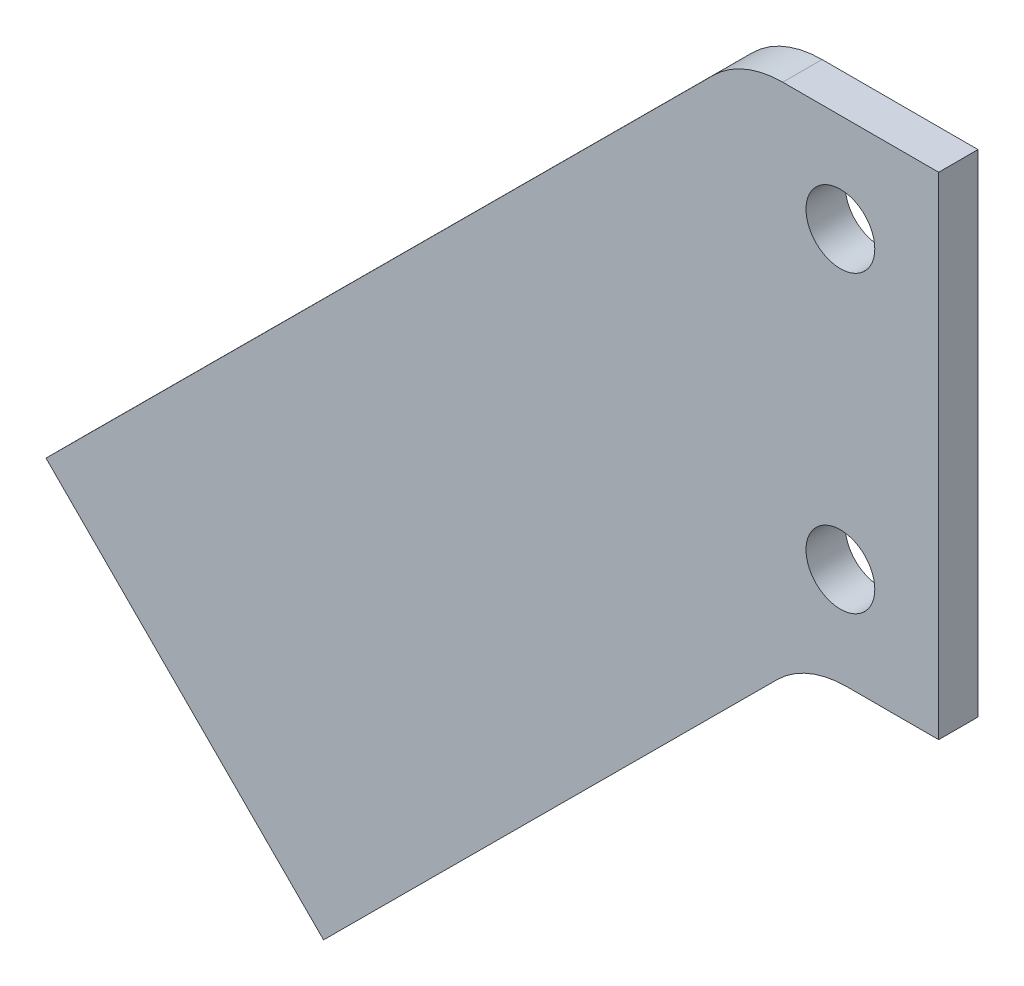
from build123d import *

# Parameters (mm, degrees)
SKETCH1_R           = 7
BOSS_EXTRUDE1_DEPTH = 8


with BuildPart() as part:
    # Sketch1 → Boss-Extrude1 (new body)
    with BuildSketch(Plane.XY):
        with BuildLine():
            Line((0, 0), (-31.73420201, 0))
            ThreePointArc((-31.73420201, 0), (-39.373295872, -1.516379008), (-45.854013577, -5.835575504))
            Line((-45.854013577, -5.835575504), (-181.644244963, -141.198115671))
            Line((-181.644244963, -141.198115671), (-125.164998695, -197.855813656))
            Line((-125.164998695, -197.855813656), (-32.854013577, -105.835575504))
            ThreePointArc((-32.854013577, -105.835575504), (-26.373295872, -101.516379008), (-18.73420201, -100))
            Line((-18.73420201, -100), (0, -100))
            Line((0, -100), (0, 0))
        make_face()
        with Locations((-20, -20)):
            Circle(SKETCH1_R, mode=Mode.SUBTRACT)
        with Locations((-20, -80)):
            Circle(SKETCH1_R, mode=Mode.SUBTRACT)
    extrude(amount=BOSS_EXTRUDE1_DEPTH)


solid = part.part
